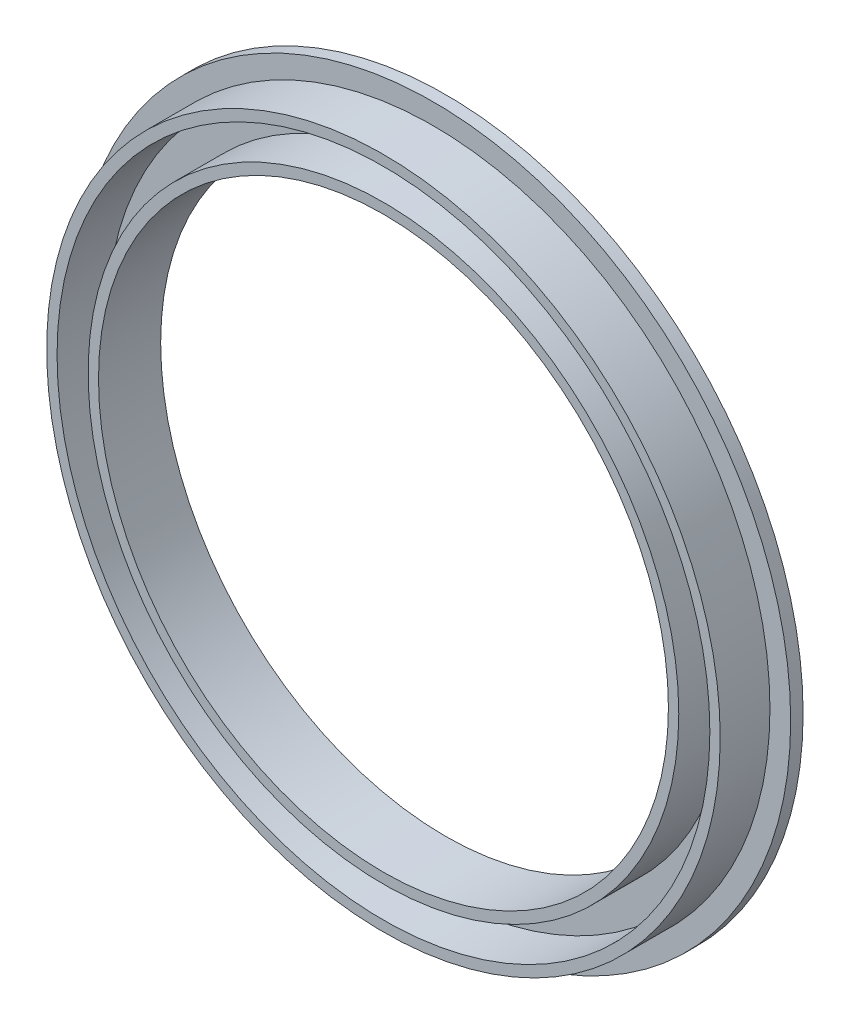
SolidWorks part; units mm, degrees
ref_plane "Front Plane" through (0, 0, 0) normal (0, 0, 1) x (1, 0, 0)
ref_plane "Top Plane" through (0, 0, 0) normal (0, 1, 0) x (1, 0, 0)
ref_plane "Right Plane" through (0, 0, 0) normal (1, 0, 0) x (0, 0, -1)
sketch "Sketch1" plane through (0, 0, 0) normal (0, 0, 1) x (1, 0, 0)
  circle A0 centre (0, 0) radius 27.5 construction
  circle A1 centre (0, 0) radius 28.5 construction
  circle A2 centre (0, 0) radius 31.5 construction
  circle A3 centre (0, 0) radius 32.5 construction
  circle A4 centre (0, 0) radius 27.5
  circle A5 centre (0, 0) radius 28.5
  circle A6 centre (0, 0) radius 31.5
  circle A7 centre (0, 0) radius 32.5
extrude "Boss-Extrude1" add sketch "Sketch1" along normal blind 6 contours A7 A6 | A5 A4
sketch "Sketch2" plane through (0, 0, 0) normal (0, 0, 1) x (1, 0, 0)
  circle A0 centre (0, 0) radius 34.5 construction
  circle A1 centre (0, 0) radius 27.5 construction
  circle A2 centre (0, 0) radius 34.5
  circle A3 centre (0, 0) radius 27.5
extrude "Boss-Extrude2" add sketch "Sketch2" along normal blind 1.2
